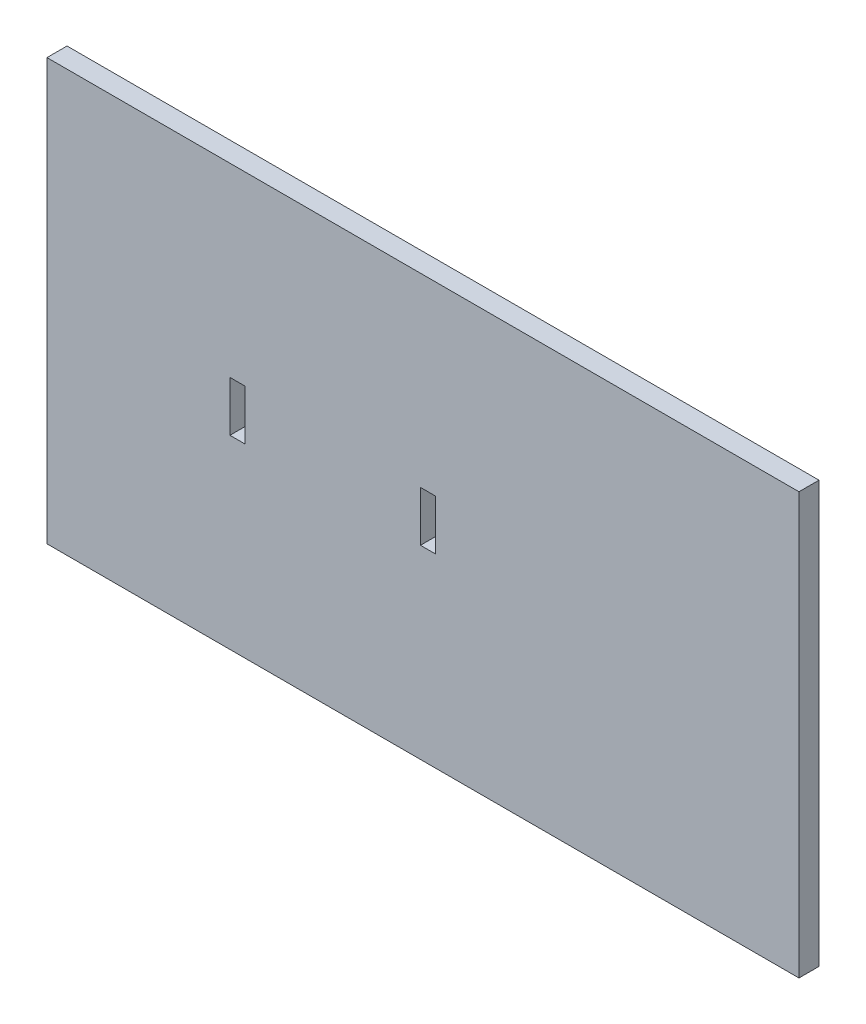
SolidWorks part; units mm, degrees
material "Q235B"
ref_plane "Front Plane" through (0, 0, 0) normal (0, 0, 1) x (1, 0, 0)
ref_plane "Top Plane" through (0, 0, 0) normal (0, 1, 0) x (1, 0, 0)
ref_plane "Right Plane" through (0, 0, 0) normal (1, 0, 0) x (0, 0, -1)
sketch "Sketch1" plane through (0, 0, 0) normal (0, 0, 1) x (1, 0, 0)
  line L1 (0, 0) -> (1500, 0)
  line L2 (0, 0) -> (0, 840)
  line L3 (0, 840) -> (1500, 840)
  line L4 (1500, 0) -> (1500, 840)
  line L5 (365, 470) -> (395, 470)
  line L6 (365, 470) -> (365, 370)
  line L7 (365, 370) -> (395, 370)
  line L8 (395, 470) -> (395, 370)
  line L9 (745, 470) -> (775, 470)
  line L10 (745, 470) -> (745, 370)
  line L11 (745, 370) -> (775, 370)
  line L12 (775, 470) -> (775, 370)
  dimension "D1" = 1500
  dimension "D2" = 840
  dimension "D3" = 365
  dimension "D4" = 745
  dimension "D5" = 30
  dimension "D6" = 30
  dimension "D7" = 100
  dimension "D8" = 100
  dimension "D9" = 370
  dimension "D10" = 370
extrude "Boss-Extrude1" add sketch "Sketch1" along normal blind 40
